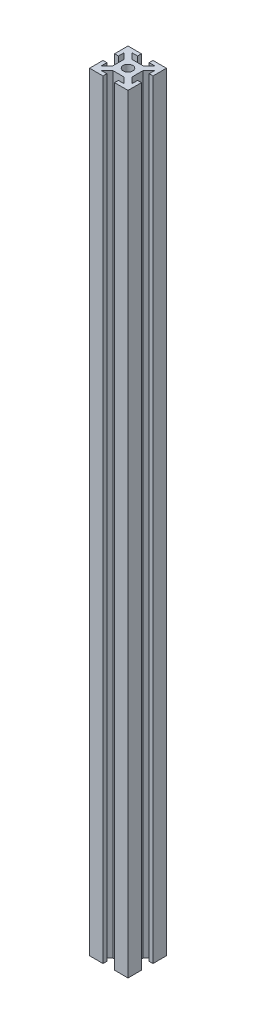
SolidWorks part; units mm, degrees
ref_plane "Front Plane" through (0, 0, 0) normal (0, 0, 1) x (1, 0, 0)
ref_plane "Top Plane" through (0, 0, 0) normal (0, 1, 0) x (1, 0, 0)
ref_plane "Right Plane" through (0, 0, 0) normal (1, 0, 0) x (0, 0, -1)
other "Configuration Table"
sketch "Sketch1" plane through (0, 0, 0) normal (0, 1, 0) x (1, 0, 0)
  line L0 (-6, 20) -> (-6, 16)
  line L5 (-20, 20) -> (-6, 20)
  line L6 (-20, 20) -> (-20, 6)
  line L7 (-20, -20) -> (-6, -20)
  line L8 (20, 20) -> (20, 6)
  line L9 (-20, 20) -> (20, -20) construction
  line L10 (-20, -20) -> (20, 20) construction
  line L11 (-6, 16) -> (-11.7574, 16)
  line L12 (-11.7574, 16) -> (-5.7574, 10)
  line L13 (5.7574, 10) -> (11.7574, 16)
  line L14 (11.7574, 16) -> (6, 16)
  line L15 (6, 16) -> (6, 20)
  line L16 (20, 6) -> (16, 6)
  line L17 (16, 6) -> (16, 11.7574)
  line L18 (16, 11.7574) -> (10, 5.7574)
  line L19 (10, -5.7574) -> (16, -11.7574)
  line L20 (16, -11.7574) -> (16, -6)
  line L21 (16, -6) -> (20, -6)
  line L22 (6, -20) -> (6, -16)
  line L23 (6, -16) -> (11.7574, -16)
  line L24 (11.7574, -16) -> (5.7574, -10)
  line L25 (-5.7574, -10) -> (-11.7574, -16)
  line L26 (-11.7574, -16) -> (-6, -16)
  line L27 (-6, -16) -> (-6, -20)
  line L28 (-20, -6) -> (-16, -6)
  line L29 (-16, -6) -> (-16, -11.7574)
  line L30 (-16, -11.7574) -> (-10, -5.7574)
  line L31 (-10, 5.7574) -> (-16, 11.7574)
  line L32 (-16, 11.7574) -> (-16, 6)
  line L33 (-16, 6) -> (-20, 6)
  line L34 (6, 20) -> (20, 20)
  line L35 (-20, -6) -> (-20, -20)
  line L36 (20, -6) -> (20, -20)
  line L37 (6, -20) -> (20, -20)
  line L39 (-5.7574, -10) -> (5.7574, -10)
  line L40 (-10, -5.7574) -> (-10, 5.7574)
  line L41 (-5.7574, 10) -> (5.7574, 10)
  line L42 (10, -5.7574) -> (10, 5.7574)
  line L43 (-10, -10) -> (10, 10) construction
  line L44 (-10, 10) -> (10, -10) construction
  circle A0 centre (0, 0) radius 5
  point P0 (0, 0)
  point P5 (0, 0)
  point P37 (0, 0)
  dimension "D10" = 10
  dimension "D1" = 40
  dimension "D2" = 4
  dimension "D3" = 4
  dimension "D4" = 14
  dimension "D5" = 14
  dimension "D6" = 3
  dimension "D7" = 3
  dimension "D8" = 4
  dimension "D9" = 20
extrude "Boss-Extrude1" add sketch "Sketch1" along normal blind 800
